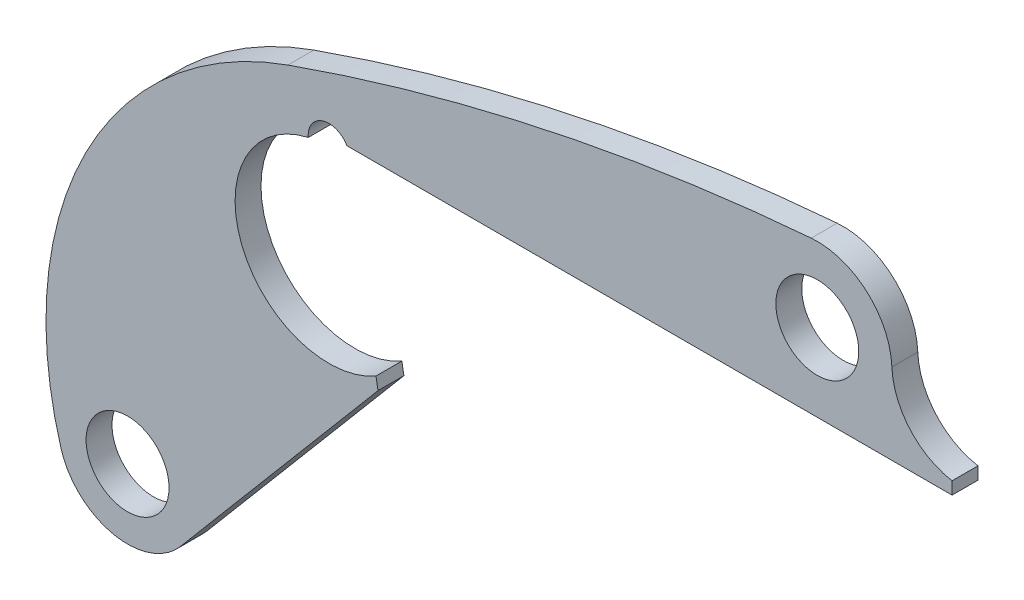
SolidWorks part; units mm, degrees
ref_plane "Front Plane" through (0, 0, 0) normal (0, 0, 1) x (1, 0, 0)
ref_plane "Top Plane" through (0, 0, 0) normal (0, 1, 0) x (1, 0, 0)
ref_plane "Right Plane" through (0, 0, 0) normal (1, 0, 0) x (0, 0, -1)
sketch "Sketch1" plane through (0, 0, 0) normal (0, 0, 1) x (1, 0, 0)
  line L0 (0, -15.3623) -> (0, 221.1323) construction
  line L1 (-64.5216, 0) -> (76.1757, 0) construction
  line L2 (-194.2, 61.7988) -> (-194.2, -422.5964) construction
  line L3 (17.3205, 100) -> (601, 100)
  line L4 (14.1583, -78.3) -> (52.573, -78.3) construction
  line L5 (-37.5291, -89.6) -> (170.8965, -89.6) construction
  line L6 (47.3, -22.5098) -> (47.3, -135.0375) construction
  line L7 (47.3, -89.6) -> (45.3802, -78.3)
  line L8 (-449.8158, -271.5) -> (226.3867, -271.5) construction
  line L9 (47.3, -89.6) -> (-143.0327, -314.754)
  line L10 (-64.5216, -191) -> (200.2329, -191) construction
  line L11 (461.2354, 175) -> (786.0535, 175) construction
  line L12 (601, 100) -> (601, 112)
  line L13 (471, 454.5963) -> (471, 132.9015) construction
  arc A0 (542.936, 178.035) -> (601, 112) centre (612.8738, 180.9856) ccw
  arc A1 (-19.9258, 88.2792) -> (45.3802, -78.3) centre (0, 0) ccw
  circle A2 centre (-194.2, -271.5) radius 40
  arc A3 (-258.4322, -290.5583) -> (-143.0327, -314.754) centre (-194.2, -271.5) ccw
  arc A4 (-39.5304, 138.9927) -> (-258.4322, -290.5583) centre (77.1093, -191) ccw
  arc A5 (542.936, 178.035) -> (465.1749, 246.764) centre (471, 175) ccw
  arc A6 (465.1749, 246.764) -> (-39.5304, 138.9927) centre (626.9821, -1746.6799) ccw
  circle A8 centre (471, 175) radius 40
  arc A9 (17.3205, 100) -> (-19.9258, 88.2792) centre (0, 90) ccw
  dimension "D3" = 20
  dimension "D4" = 181
  dimension "D1" = 90
  dimension "D10" = 80
  dimension "D11" = 134
  dimension "D13" = 700
  dimension "D14" = 175
  dimension "D16" = 144
  dimension "D17" = 4000
  dimension "D20" = 140
  dimension "D21" = 80
  dimension "D2" = 100
  dimension "D5" = 78.3
  dimension "D6" = 89.6
  dimension "D7" = 47.3
  dimension "D8" = 271.5
  dimension "D9" = 194.2
  dimension "D12" = 191
  dimension "D15" = 471
  dimension "D18" = 601
  dimension "D19" = 12
extrude "Boss-Extrude1" add sketch "Sketch1" along normal blind 25
